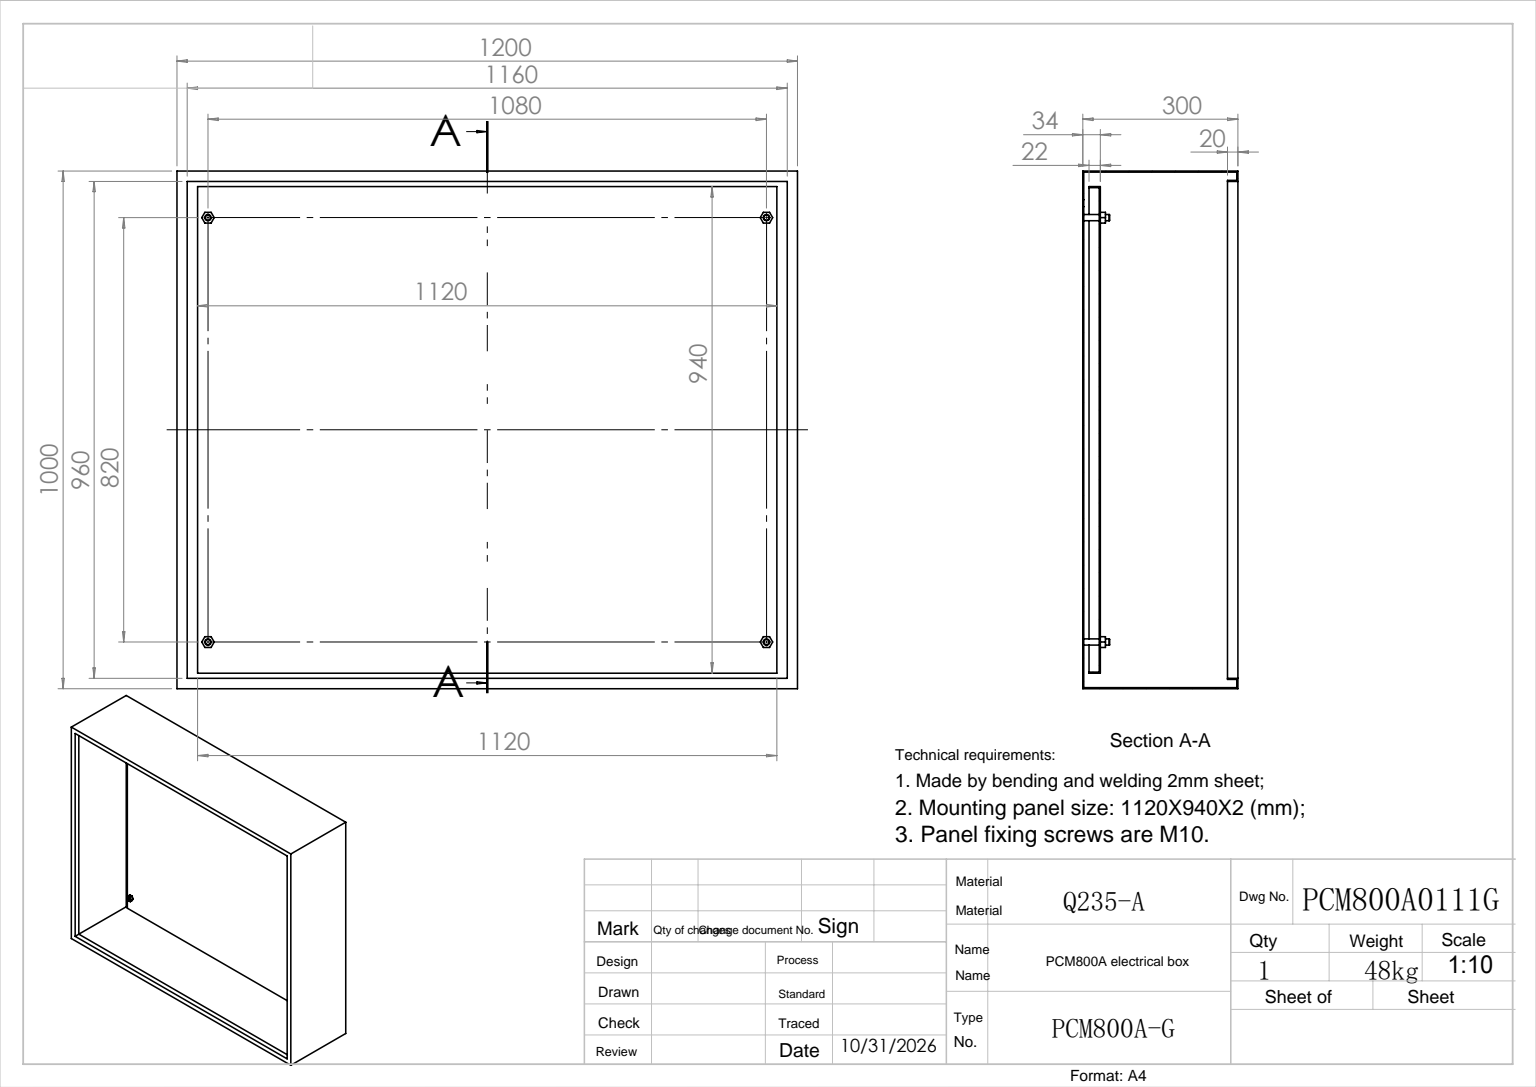
SolidWorks part; units mm, degrees
ref_plane "前视基准面" through (0, 0, 0) normal (0, 0, 1) x (1, 0, 0)
ref_plane "上视基准面" through (0, 0, 0) normal (0, 1, 0) x (1, 0, 0)
ref_plane "右视基准面" through (0, 0, 0) normal (1, 0, 0) x (0, 0, -1)
sketch "草图1" plane through (0, 0, 0) normal (0, 0, 1) x (1, 0, 0)
  line L1 (0, 0) -> (1200, 0)
  line L2 (0, 0) -> (0, -1000)
  line L3 (0, -1000) -> (1200, -1000)
  line L4 (1200, 0) -> (1200, -1000)
  dimension "D1" = 1200
  dimension "D2" = 1000
extrude "凸台-拉伸1" add sketch "草图1" along normal blind 300
shell "抽壳1" thickness 2
sketch "草图2" plane through (0, 0, 2) normal (0, 0, 1) x (1, 0, 0)
  line L0 (1198, -2) -> (2, -2) construction
  line L1 (0, 0) -> (0, -1000) construction
  circle A0 centre (60, -62) radius 7
  dimension "D1" = 14
  dimension "D2" = 60
  dimension "D3" = 60
extrude "切除-拉伸1" cut sketch "草图2" against normal through all
pattern_linear "阵列(线性)1" count 3 spacing 388 along (0, -1, 0) of "切除-拉伸1"
pattern_linear "阵列(线性)2" count 3 spacing 538 along (1, 0, 0) of "切除-拉伸1"
sketch "草图3" plane through (0, 0, 300) normal (0, 0, 1) x (1, 0, 0)
  line L0 (1200, 0) -> (0, 0) construction
  line L1 (1200, 0) -> (0, 0)
  line L2 (0, 0) -> (0, -1000) construction
  line L3 (0, -1000) -> (1200, -1000) construction
  line L4 (1200, -1000) -> (1200, 0) construction
  line L5 (0, 0) -> (0, -1000)
  line L6 (0, -1000) -> (1200, -1000)
  line L7 (1200, -1000) -> (1200, 0)
  line L8 (1180, -20) -> (20, -20)
  line L9 (20, -20) -> (20, -980)
  line L10 (20, -980) -> (1180, -980)
  line L11 (1180, -980) -> (1180, -20)
  dimension "D1" = 20
extrude "凸台-拉伸2" add sketch "草图3" against normal blind 2
sketch "草图4" plane through (0, 0, 300) normal (0, 0, 1) x (1, 0, 0)
  line L0 (18, -18) -> (18, -982)
  line L1 (20, -20) -> (1180, -20)
  line L2 (20, -20) -> (20, -980)
  line L3 (20, -980) -> (1180, -980)
  line L4 (1180, -20) -> (1180, -980)
  line L5 (18, -982) -> (1182, -982)
  line L6 (1182, -18) -> (1182, -982)
  line L7 (18, -18) -> (1182, -18)
  dimension "D1" = 2
extrude "凸台-拉伸3" add sketch "草图4" against normal blind 20
sketch "草图5" plane through (0, 0, 2) normal (0, 0, 1) x (1, 0, 0)
  line L0 (1180, -20) -> (20, -20) construction
  line L1 (40, -30) -> (1160, -30)
  line L2 (40, -30) -> (40, -970)
  line L3 (40, -970) -> (1160, -970)
  line L4 (1160, -30) -> (1160, -970)
  line L5 (20, -980) -> (1180, -980) construction
  line L6 (20, -20) -> (20, -980) construction
  line L7 (1180, -980) -> (1180, -20) construction
  dimension "D1" = 10
  dimension "D2" = 10
  dimension "D3" = 20
  dimension "D4" = 20
extrude "凸台-拉伸4" add sketch "草图5" along normal blind 2 from offset 30 separate body
sketch "草图6" plane through (0, 0, 34) normal (0, 0, 1) x (1, 0, 0)
  line L0 (1160, -970) -> (1160, -30) construction
  line L1 (40, -30) -> (1160, -30)
  line L2 (40, -30) -> (40, -970)
  line L3 (40, -970) -> (1160, -970)
  line L4 (1160, -30) -> (1160, -970)
  line L5 (40, -970) -> (1160, -970) construction
  line L6 (42, -32) -> (42, -968)
  line L7 (42, -968) -> (1158, -968)
  line L8 (1158, -32) -> (1158, -968)
  line L9 (42, -32) -> (1158, -32)
  dimension "D1" = 2
extrude "凸台-拉伸5" add sketch "草图6" against normal blind 22
sketch "草图8" plane through (0, 0, 2) normal (0, 0, 1) x (1, 0, 0)
  line L0 (1160, -30) -> (40, -30) construction
  line L1 (40, -30) -> (40, -970) construction
  circle A0 centre (60, -90) radius 6
  dimension "D1" = 12
  dimension "D2" = 60
  dimension "D3" = 20
extrude "凸台-拉伸6" add sketch "草图8" along normal blind 50
fillet "圆角1" radius 1 1 edges at (66, -90, 52)
sketch "草图9" plane through (0, 0, 34) normal (0, 0, 1) x (1, 0, 0)
  line L1 (66, -79.6077) -> (54, -79.6077)
  line L2 (54, -79.6077) -> (48, -90)
  line L3 (48, -90) -> (54, -100.3923)
  line L4 (54, -100.3923) -> (66, -100.3923)
  line L5 (66, -100.3923) -> (72, -90)
  line L6 (72, -90) -> (66, -79.6077)
  circle A0 centre (60, -90) radius 10.3923 construction
  dimension "D1" = 12
extrude "凸台-拉伸7" add sketch "草图9" along normal blind 10
pattern_linear "阵列(线性)4" count 2 spacing 1080 along (1, 0, 0) count 2 spacing 820 along (0, -1, 0) of "凸台-拉伸7", "圆角1", "凸台-拉伸6"
